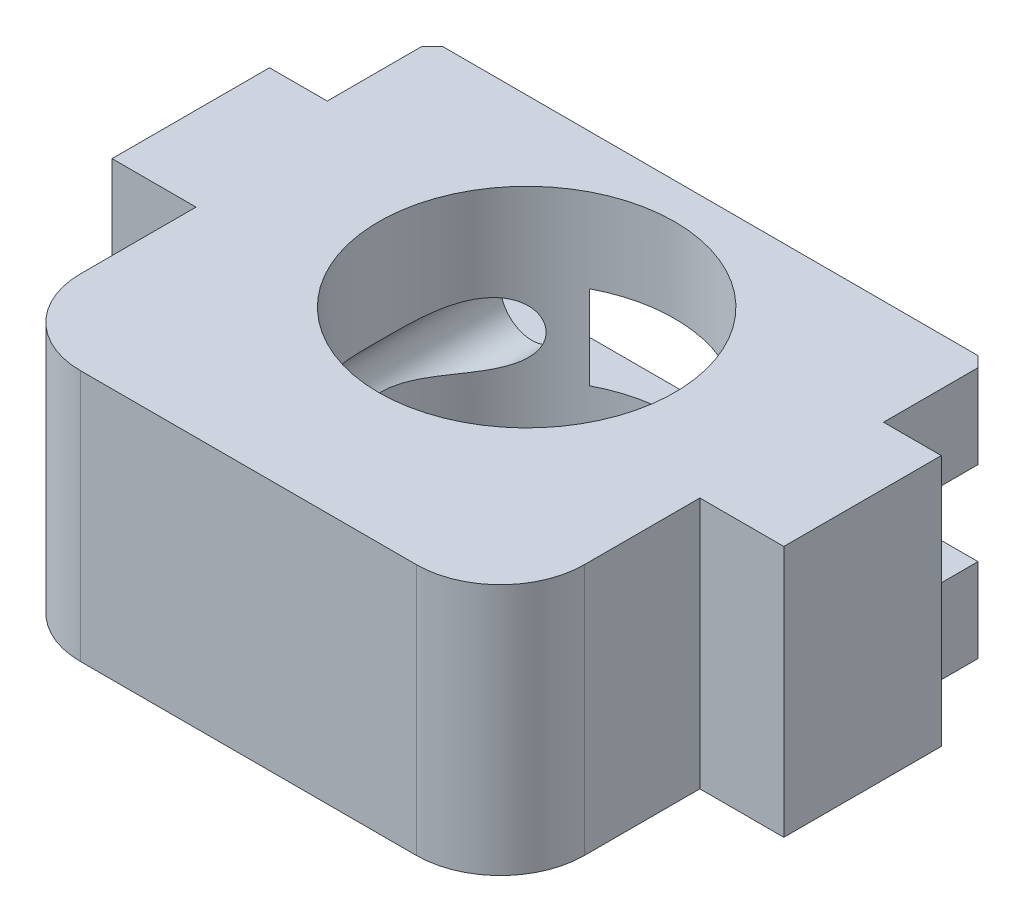
from build123d import *

# Parameters (mm, degrees)
BOSS_EXTRUDE1_DEPTH = 24
SKETCH2_W           = 5
SKETCH2_H           = 8
CUT_EXTRUDE1_DEPTH  = 64
SKETCH3_R           = 3
CUT_EXTRUDE2_DEPTH  = 35
SKETCH4_R           = 14.1
CUT_EXTRUDE3_DEPTH  = 35
CHAMFER1_SIZE       = 1
CHAMFER2_SIZE       = 3


with BuildPart() as part:
    # Sketch1 → Boss-Extrude1 (new body)
    with BuildSketch(Plane(origin=(0, 0, 0), x_dir=(1, 0, 0), z_dir=(0, 1, 0))):
        with BuildLine():
            Line((-24, 19), (-24, 8))
            ThreePointArc((-24, 8), (-21.656854249, 2.343145751), (-16, 0))
            Line((-16, 0), (16, 0))
            ThreePointArc((16, 0), (21.656854249, 2.343145751), (24, 8))
            Line((24, 8), (24, 19))
            Line((24, 19), (32, 19))
            Line((32, 19), (32, 34))
            Line((32, 34), (26.5, 34))
            Line((26.5, 34), (26.5, 44))
            Line((26.5, 44), (-26.5, 44))
            Line((-26.5, 44), (-26.5, 34))
            Line((-26.5, 34), (-32, 34))
            Line((-32, 34), (-32, 19))
            Line((-32, 19), (-24, 19))
        make_face()
    extrude(amount=BOSS_EXTRUDE1_DEPTH)

    # Sketch2 → Cut-Extrude1 (cut)
    with BuildSketch(Plane.ZY.offset(26.5)):
        with Locations((-41.5, 12)):
            Rectangle(SKETCH2_W, SKETCH2_H)
    extrude(amount=-CUT_EXTRUDE1_DEPTH, mode=Mode.SUBTRACT)

    # Sketch3 → Cut-Extrude2 (cut)
    with BuildSketch(Plane(origin=(0, 0, -39), x_dir=(-1, 0, 0), z_dir=(0, 0, -1))):
        with Locations((-12, 12)):
            Circle(SKETCH3_R)
        with Locations(Location((12, 12, 0), (0, 0, 180))):
            Circle(SKETCH3_R)
    extrude(amount=-CUT_EXTRUDE2_DEPTH, mode=Mode.SUBTRACT)

    # Sketch4 → Cut-Extrude3 (cut)
    with BuildSketch(Plane.XZ):
        with Locations(Location((0, -26.5, 0), (0, 0, 270))):
            Circle(SKETCH4_R)
    extrude(amount=-CUT_EXTRUDE3_DEPTH, mode=Mode.SUBTRACT)

    # Chamfer1
    chamfer1_edges = [part.edges().sort_by_distance(p)[0] for p in [
        (-26.5, 20, -44),
        (26.5, 20, -44),
        (-26.5, 4, -44),
        (26.5, 4, -44),
        (0, 8, -44),
        (0, 16, -44),
    ]]
    chamfer(chamfer1_edges, length=CHAMFER1_SIZE)

    # Chamfer2
    chamfer2_edges = [part.edges().sort_by_distance(p)[0] for p in [
        (0, 0, -12.4),
    ]]
    chamfer(chamfer2_edges, length=CHAMFER2_SIZE)


solid = part.part
